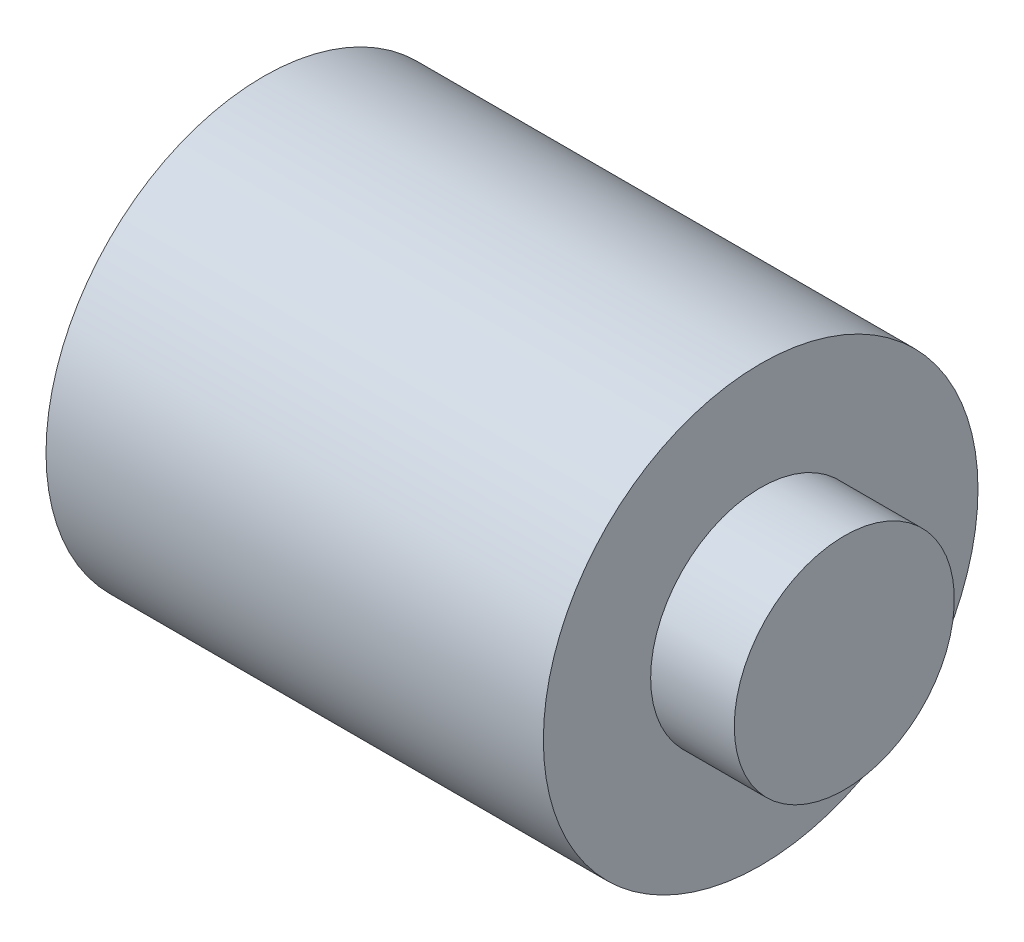
SolidWorks part; units mm, degrees
ref_plane "前视基准面" through (0, 0, 0) normal (0, 0, 1) x (1, 0, 0)
ref_plane "上视基准面" through (0, 0, 0) normal (0, 1, 0) x (1, 0, 0)
ref_plane "右视基准面" through (0, 0, 0) normal (1, 0, 0) x (0, 0, -1)
sketch "草图1" plane through (0, 0, 0) normal (1, 0, 0) x (0, 0, -1)
  circle A0 centre (0, 0) radius 19.75
  dimension "D1" = 39.5
extrude "凸台-拉伸1" add sketch "草图1" along normal blind 45.2
sketch "草图2" plane through (45.2, 0, 0) normal (1, 0, 0) x (0, 0, -1)
  circle A0 centre (0, 0) radius 10
  dimension "D1" = 20
extrude "凸台-拉伸2" add sketch "草图2" along normal blind 7.6
